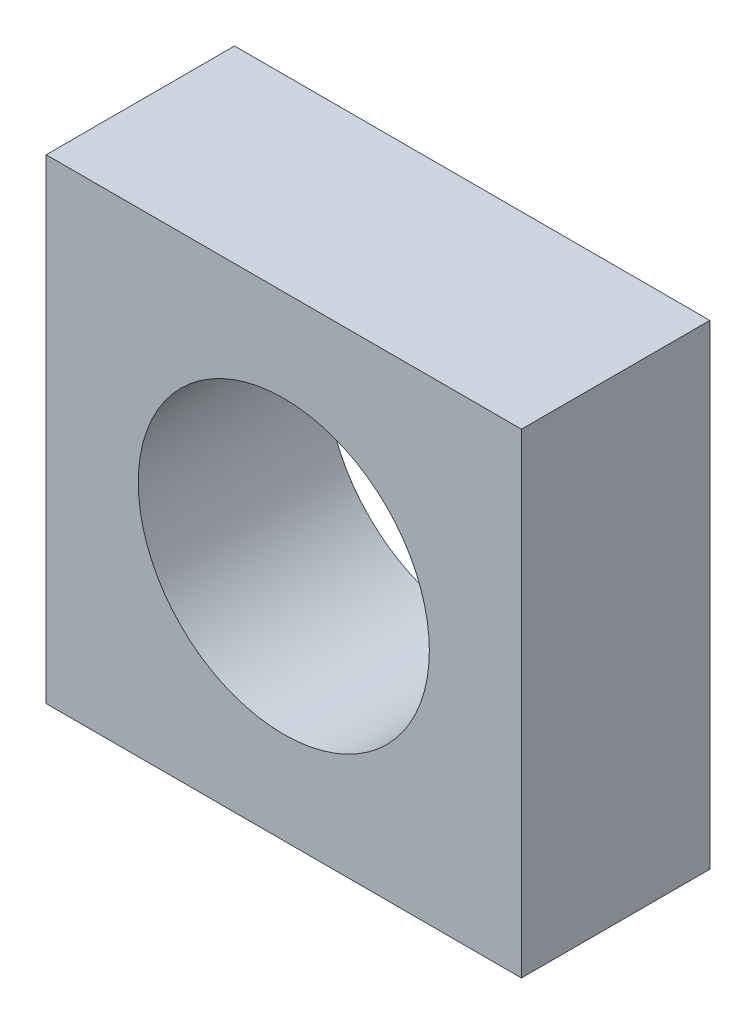
SolidWorks part; units mm, degrees
ref_plane "Front Plane" through (0, 0, 0) normal (0, 0, 1) x (1, 0, 0)
ref_plane "Top Plane" through (0, 0, 0) normal (0, 1, 0) x (1, 0, 0)
ref_plane "Right Plane" through (0, 0, 0) normal (1, 0, 0) x (0, 0, -1)
other "Configuration Table"
sketch "Sketch1" plane through (0, 0, 0) normal (0, 0, 1) x (1, 0, 0)
  line L4 (13.5518, -4.1634) -> (25.5518, -4.1634)
  line L5 (25.5518, 7.8366) -> (13.5518, 7.8366)
  line L6 (25.5518, -4.1634) -> (25.5518, 7.8366)
  line L7 (13.5518, 7.8366) -> (13.5518, -4.1634)
  circle A2 centre (19.5518, 1.8366) radius 3.6746
extrude "Boss-Extrude1" add sketch "Sketch1" along normal up to surface (4.756 mm away)
